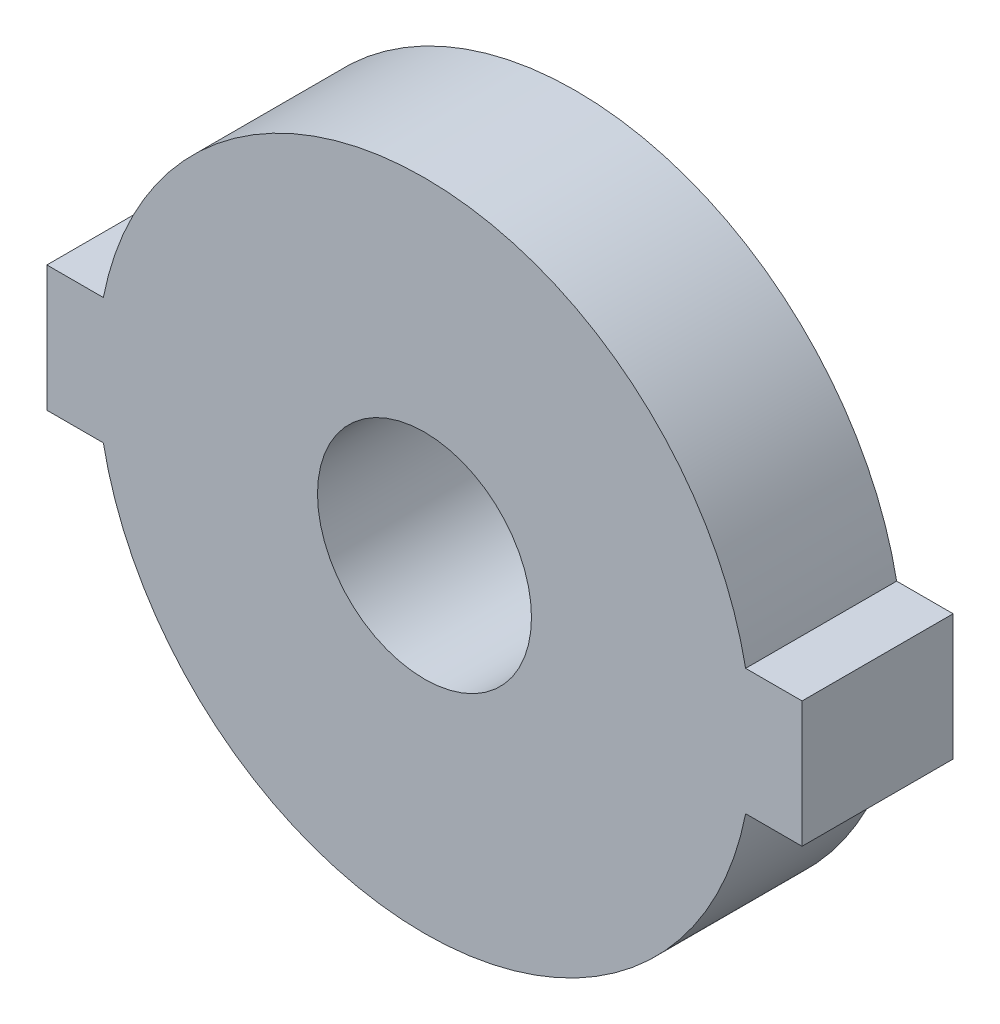
from build123d import *

# Parameters (mm, degrees)
SKETCH1_R           = 4.25
BOSS_EXTRUDE1_DEPTH = 6


with BuildPart() as part:
    # Sketch1 → Boss-Extrude1 (new body)
    with BuildSketch(Plane.XY.offset(6)):
        with BuildLine():
            Line((-12.757350822, 2.5), (-15, 2.5))
            Line((-15, 2.5), (-15, -2.5))
            Line((-15, -2.5), (-12.757350822, -2.5))
            ThreePointArc((-12.757350822, -2.5), (0, -13), (12.757350822, -2.5))
            Line((12.757350822, -2.5), (15, -2.5))
            Line((15, -2.5), (15, 2.5))
            Line((15, 2.5), (12.757350822, 2.5))
            ThreePointArc((12.757350822, 2.5), (0, 13), (-12.757350822, 2.5))
        make_face()
        with Locations(Location((0, 0, 0), (0, 0, 180))):
            Circle(SKETCH1_R, mode=Mode.SUBTRACT)
    extrude(amount=-BOSS_EXTRUDE1_DEPTH)


solid = part.part
